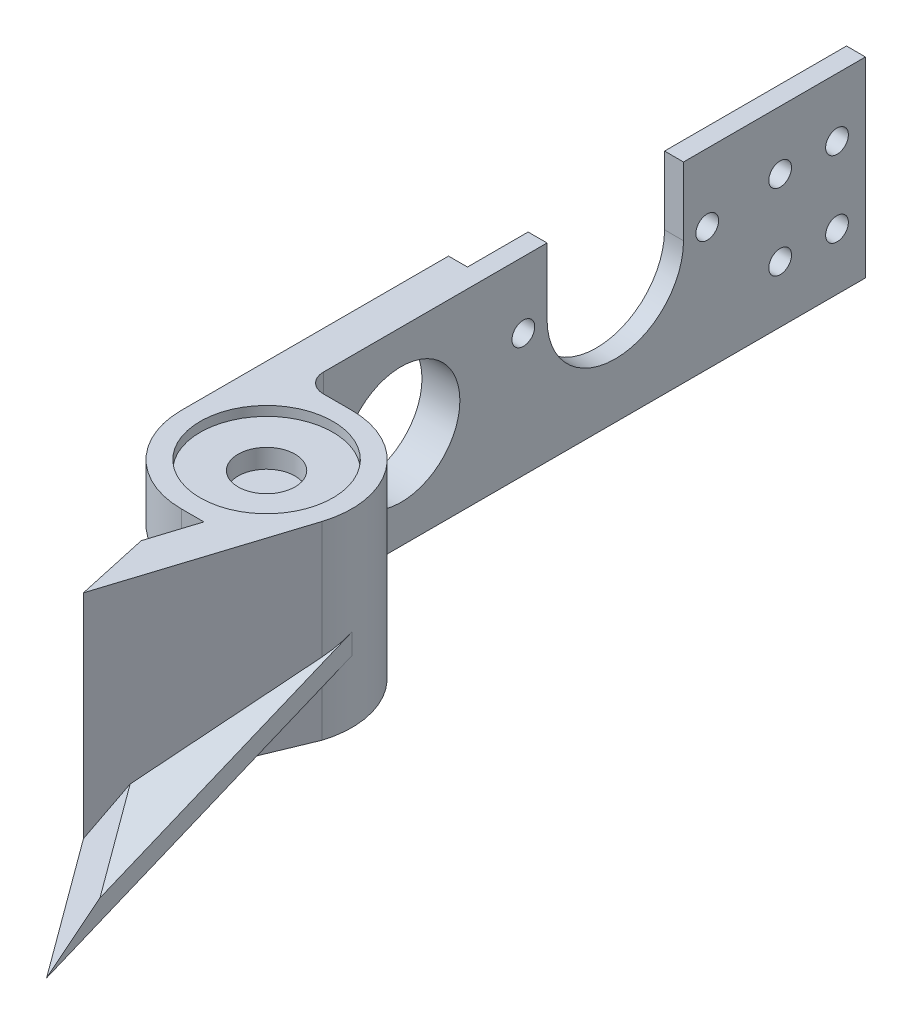
from build123d import *

# Parameters (mm, degrees)
SKETCH_1_W                  = 90
SKETCH_1_H                  = 100
SKETCH_1_R                  = 31
EXTRUDE_1_DEPTH             = 20
EXTRUDE_2_DEPTH             = 30
EXTRUDE_3_REACH             = 183.331
EXTRUDE_3_DIRECTION_2_REACH = 183.331
EXTRUDE_4_DEPTH             = 100
CUT_EXTRUDE_1_DEPTH         = 100
CUT_EXTRUDE_1_DEPTH_BACK    = 70
CUT_EXTRUDE_2_DEPTH         = 100
EXTRUDE_6_REACH             = 292.174
CUT_EXTRUDE_3_REACH         = 339.181
SKETCH_9_R                  = 35
CUT_EXTRUDE_4_DEPTH         = 5
SKETCH_10_R                 = 15
CUT_EXTRUDE_5_DEPTH         = 10
HOLE_WIZARD_M6_1_D          = 5
HOLE_WIZARD_M6_1_DEPTH      = 15
HOLE_WIZARD_M6_1_TIP        = 1.502151548
SKETCH_15_W                 = 20
SKETCH_15_H                 = 100
EXTRUDE_7_DEPTH             = 6
SKETCH_16_R                 = 6
EXTRUDE_8_DEPTH             = 10


with BuildPart() as part:
    # 草图1 → 凸台-拉伸1 (new body)
    with BuildSketch(Plane(origin=(0, 0, 0), x_dir=(0, 0, -1), z_dir=(1, 0, 0))):
        with Locations((-6, -1)):
            Rectangle(SKETCH_1_W, SKETCH_1_H)
        Circle(SKETCH_1_R, mode=Mode.SUBTRACT)
    extrude(amount=EXTRUDE_1_DEPTH)

    # 草图2 → 凸台-拉伸2 (add)
    with BuildSketch(Plane(origin=(0, 49, 0), x_dir=(1, 0, 0), z_dir=(0, 1, 0))):
        with BuildLine():
            Line((0, -51), (0, -96))
            ThreePointArc((0, -96), (13.180194847, -127.819805153), (45, -141))
            Line((45, -141), (76.819805153, -141))
            Line((76.819805153, -141), (76.819805153, -127.819805153))
            ThreePointArc((76.819805153, -127.819805153), (86.574578963, -78.779245544), (45, -51))
            Line((45, -51), (30, -51))
            ThreePointArc((30, -51), (22.928932188, -48.071067812), (20, -41))
            Line((20, -41), (0, -41))
            Line((0, -41), (0, -51))
        make_face()
    extrude(amount=-EXTRUDE_2_DEPTH)

    # 凸台-拉伸3: up to this face of the body (flat: up to its plane)
    extrude_3_end = Plane(part.part.faces().sort_by_distance((36.366131186, 49, 76.243712536))[0])
    # 草图3 → 凸台-拉伸3 (add, up to the picked face)
    with BuildSketch(Plane.XZ.offset(-19), mode=Mode.PRIVATE) as extrude_3_sk1:
        with BuildLine():
            Line((20, 71), (45, 71))
            ThreePointArc((45, 71), (65.17535119, 81.23669399), (68.828390679, 103.563583652))
            Line((68.828390679, 103.563583652), (48.974479643, 166.111546424))
            Line((48.974479643, 166.111546424), (57.556783249, 205.18))
            Line((57.556783249, 205.18), (87.891103222, 109.614450573))
            ThreePointArc((87.891103222, 109.614450573), (81.315632142, 69.426049181), (45, 51))
            Line((45, 51), (40, 51))
            Line((40, 51), (30, 51))
            ThreePointArc((30, 51), (22.928932188, 48.071067812), (20, 41))
            Line((20, 41), (0, 41))
            Line((0, 41), (0, 51))
            ThreePointArc((0, 51), (5.857864376, 65.142135624), (20, 71))
        make_face()
    extrude_3_tool1 = split(extrude(extrude_3_sk1.sketch, amount=-EXTRUDE_3_REACH, mode=Mode.PRIVATE), bisect_by=extrude_3_end, keep=Keep.BOTH, mode=Mode.PRIVATE)
    add(extrude_3_tool1.solids().sort_by(Axis((7.18178, 19, 63.81822), (0, 1, 0)))[0])

    # 凸台-拉伸3 direction 2: up to this face of the body (flat: up to its plane)
    extrude_3_direction_2_end = Plane(part.part.faces().sort_by_distance((10, -51, 6))[0])
    # 草图3 → 凸台-拉伸3 direction 2 (add, up to the picked face)
    with BuildSketch(Plane.XZ.offset(-19), mode=Mode.PRIVATE) as extrude_3_direction_2_sk1:
        with BuildLine():
            Line((20, 71), (45, 71))
            ThreePointArc((45, 71), (65.17535119, 81.23669399), (68.828390679, 103.563583652))
            Line((68.828390679, 103.563583652), (48.974479643, 166.111546424))
            Line((48.974479643, 166.111546424), (57.556783249, 205.18))
            Line((57.556783249, 205.18), (87.891103222, 109.614450573))
            ThreePointArc((87.891103222, 109.614450573), (81.315632142, 69.426049181), (45, 51))
            Line((45, 51), (40, 51))
            Line((40, 51), (30, 51))
            ThreePointArc((30, 51), (22.928932188, 48.071067812), (20, 41))
            Line((20, 41), (0, 41))
            Line((0, 41), (0, 51))
            ThreePointArc((0, 51), (5.857864376, 65.142135624), (20, 71))
        make_face()
    extrude_3_direction_2_tool1 = split(extrude(extrude_3_direction_2_sk1.sketch, amount=EXTRUDE_3_DIRECTION_2_REACH, mode=Mode.PRIVATE), bisect_by=extrude_3_direction_2_end, keep=Keep.BOTH, mode=Mode.PRIVATE)
    add(extrude_3_direction_2_tool1.solids().sort_by(Axis((7.18178, 19, 63.81822), (0, -1, 0)))[0])

    # 草图4 → 凸台-拉伸4 (add)
    with BuildSketch(Plane.ZY):
        Polygon((79.044272811, -11.09336582), (82.871107135, -1.854570495), (260.927976749, -75.608140763), (257.101142425, -84.846936088), align=None)
    extrude(amount=-EXTRUDE_4_DEPTH)

    # 草图5 → 切除-拉伸1 (cut, two sides: drawn at the far end of the back side and taken through both)
    with BuildSketch(Plane.XZ.offset(51).offset(-CUT_EXTRUDE_1_DEPTH_BACK)):
        with BuildLine():
            Line((90, 273.997870748), (90, 257.101142425))
            Line((90, 257.101142425), (90, 96))
            ThreePointArc((90, 96), (89.163059449, 87.361471182), (86.683369771, 79.044272811))
            Line((86.683369771, 79.044272811), (109.692797529, 79.044272811))
            Line((109.692797529, 79.044272811), (210.132802407, 79.044272811))
            Line((210.132802407, 79.044272811), (210.132802407, 273.997870748))
            Line((210.132802407, 273.997870748), (90, 273.997870748))
        make_face()
        with BuildLine():
            Line((-30.73238043, 79.044272811), (63.371263307, 79.044272811))
            ThreePointArc((63.371263307, 79.044272811), (69.402906592, 90.568780078), (68.828390679, 103.563583652))
            Line((68.828390679, 103.563583652), (48.974479643, 166.111546424))
            Line((48.974479643, 166.111546424), (51.012141043, 175.387410276))
            Line((51.012141043, 175.387410276), (57.556783249, 205.18))
            Line((57.556783249, 205.18), (90, 257.101142425))
            Line((90, 257.101142425), (-30.73238043, 295.986256779))
            Line((-30.73238043, 295.986256779), (-30.73238043, 79.044272811))
        make_face()
    extrude(amount=CUT_EXTRUDE_1_DEPTH + CUT_EXTRUDE_1_DEPTH_BACK, mode=Mode.SUBTRACT)


with BuildPart() as body_2:
    # of the pieces the cut leaves, the one that is kept (cut_extrude_1_keep)
    add(part.part.solids().sort_by_distance((0, 49, 96))[0])

    # 草图6 → 切除-拉伸2 (cut)
    with BuildSketch(Plane(origin=(90, 0, 0), x_dir=(0, 0, -1), z_dir=(1, 0, 0))):
        Polygon((-109.614450573, -51), (-166.111546424, -47.15781139), (-175.387410276, -51), align=None)
    extrude(amount=-CUT_EXTRUDE_2_DEPTH, mode=Mode.SUBTRACT)

    # 凸台-拉伸6: up to this face of the body (flat: up to its plane)
    extrude_6_end = Plane(body_2.part.faces().sort_by_distance((79.164953254, -45.54677493, 188.353419651))[0])
    # 草图7 → 凸台-拉伸6 (add, up to the picked face)
    with BuildSketch(Plane.XZ.offset(51), mode=Mode.PRIVATE) as extrude_6_sk1:
        Polygon((57.556783249, 205.18), (58.718959047, 201.518669574), (56.75248601, 201.518669574), align=None)
    extrude_6_tool1 = split(extrude(extrude_6_sk1.sketch, amount=EXTRUDE_6_REACH, mode=Mode.PRIVATE), bisect_by=extrude_6_end, keep=Keep.BOTH, mode=Mode.PRIVATE)
    add(extrude_6_tool1.solids().sort_by(Axis((57.676076, -51, 202.739113), (0, -1, 0)))[0])

    # 切除-拉伸3: up to this plane
    cut_extrude_3_end = Plane(origin=(57.556783249, 236.229998665, 205.18), z_dir=(0.9531356271558171, 0, 0.3025433460618284))
    # 草图8 → 切除-拉伸3 (cut, up to the surface)
    with BuildSketch(Plane(origin=(90, -84.846936088, 257.101142425), x_dir=(-0.8660475161032836, -0.19132705878879122, 0.46190438017685376), z_dir=(-0.4999616983843192, 0.3314220360536652, -0.8001235743100625)), mode=Mode.PRIVATE) as cut_extrude_3_sk1:
        Polygon((0, 0), (-39.725764101, 22.935680597), (0, 22.935680597), align=None)
    cut_extrude_3_tool1 = split(extrude(cut_extrude_3_sk1.sketch, amount=CUT_EXTRUDE_3_REACH, mode=Mode.PRIVATE), bisect_by=cut_extrude_3_end, keep=Keep.BOTH, mode=Mode.PRIVATE)
    add(cut_extrude_3_tool1.solids().sort_by_distance((101.468133, -68.186861, 256.836044))[0], mode=Mode.SUBTRACT)

    # 草图9 → 切除-拉伸4 (cut)
    with BuildSketch(Plane(origin=(0, 49, 0), x_dir=(1, 0, 0), z_dir=(0, 1, 0))):
        with Locations(Location((45, -96, 0), (0, 0, 270))):
            Circle(SKETCH_9_R)
    extrude(amount=-CUT_EXTRUDE_4_DEPTH, mode=Mode.SUBTRACT)

    # 草图10 → 切除-拉伸5 (cut)
    with BuildSketch(Plane(origin=(0, 44, 0), x_dir=(1, 0, 0), z_dir=(0, 1, 0))):
        with Locations(Location((45, -96, 0), (0, 0, 270))):
            Circle(SKETCH_10_R)
    extrude(amount=-CUT_EXTRUDE_5_DEPTH, mode=Mode.SUBTRACT)

    # M6 螺纹孔1
    with Locations(Plane.ZY):
        with Locations((28.991378029, 28.991378029), (-28.991378029, 28.991378029), (-28.991378029, -28.991378029), (28.991378029, -28.991378029)):
            Hole(HOLE_WIZARD_M6_1_D / 2, depth=HOLE_WIZARD_M6_1_DEPTH)
            with Locations((0, 0, -(HOLE_WIZARD_M6_1_DEPTH + HOLE_WIZARD_M6_1_TIP / 2))):  # 118° drill point
                Cone(0, HOLE_WIZARD_M6_1_D / 2, HOLE_WIZARD_M6_1_TIP, mode=Mode.SUBTRACT)

    # 草图15 → 凸台-拉伸7 (add)
    with BuildSketch(Plane(origin=(0, 0, -39), x_dir=(-1, 0, 0), z_dir=(0, 0, -1))):
        with Locations((-10, -1)):
            Rectangle(SKETCH_15_W, SKETCH_15_H)
    extrude(amount=EXTRUDE_7_DEPTH)

    # 草图16 → 凸台-拉伸8 (add)
    with BuildSketch(Plane(origin=(20, 0, 0), x_dir=(0, 0, -1), z_dir=(1, 0, 0))):
        with BuildLine():
            Line((45, -51), (73, -51))
            Line((73, -51), (245, -51))
            Line((245, -51), (245, 49.999994373))
            Line((245, 49.999994373), (148.999999307, 49.999994373))
            Line((148.999999307, 49.999994373), (148.999999307, 13.999994373))
            ThreePointArc((148.999999307, 13.999994373), (112.999999307, -22.000005627), (76.999999307, 13.999994373))
            Line((76.999999307, 13.999994373), (76.999999307, 49))
            Line((76.999999307, 49), (73, 49))
            Line((73, 49), (45, 49))
            Line((45, 49), (45, -51))
        make_face()
        with Locations((230, 19)):
            Circle(SKETCH_16_R, mode=Mode.SUBTRACT)
        with Locations((200, 19)):
            Circle(SKETCH_16_R, mode=Mode.SUBTRACT)
        with Locations((230, -21)):
            Circle(SKETCH_16_R, mode=Mode.SUBTRACT)
        with Locations((200, -21)):
            Circle(SKETCH_16_R, mode=Mode.SUBTRACT)
        with Locations((161.499999307, 13.999994373)):
            Circle(SKETCH_16_R, mode=Mode.SUBTRACT)
        with Locations((64.499999307, 13.999994373)):
            Circle(SKETCH_16_R, mode=Mode.SUBTRACT)
    extrude(amount=-EXTRUDE_8_DEPTH)


solid = body_2.part
